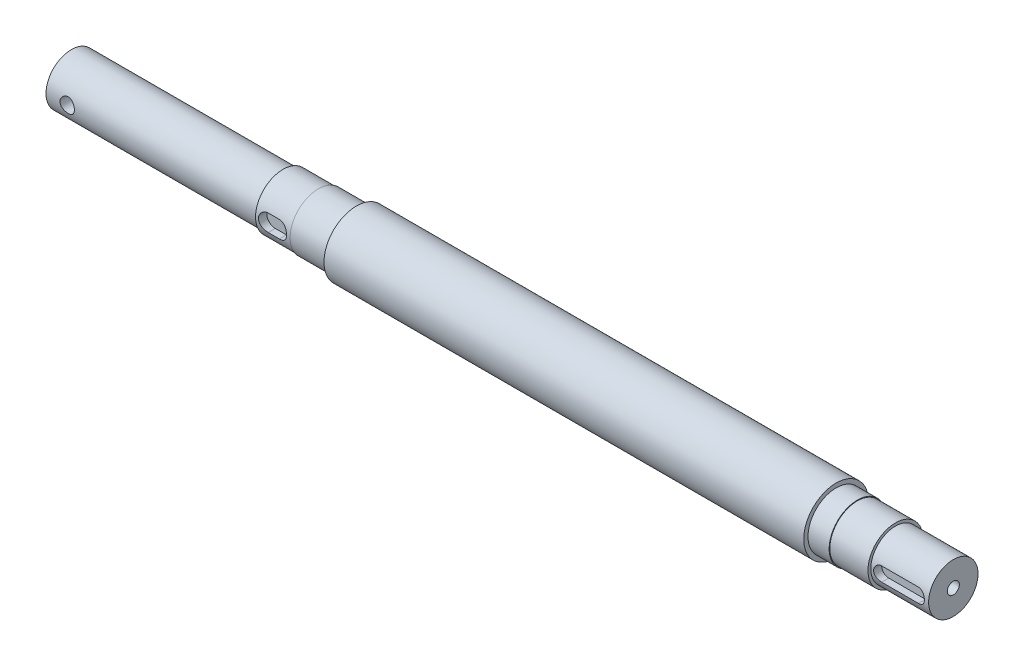
from build123d import *

# Parameters (mm, degrees)
SKETCH_1_R               = 23
EXTRUDE_1_DEPTH          = 340
SKETCH_2_R               = 20
EXTRUDE_2_DEPTH          = 27
SKETCH_3_R               = 19.5
EXTRUDE_3_DEPTH          = 25
EXTRUDE_START            = 15
SKETCH_4_R               = 20
EXTRUDE_4_DEPTH          = 15
EXTRUDE_START_2          = 27
SKETCH_5_R               = 19.5
EXTRUDE_5_DEPTH          = 27
SKETCH_6_R               = 17.5
EXTRUDE_6_DEPTH          = 41
CUT_EXTRUDE_1_DEPTH      = 5.73
SKETCH_8_R               = 18
EXTRUDE_7_DEPTH          = 150
HOLE_WIZARD_M12_2_D      = 10.2
HOLE_WIZARD_M12_2_DEPTH  = 20
HOLE_WIZARD_M12_2_TIP    = 3.064389157
HOLE_WIZARD_M10_1_D      = 8.5
HOLE_WIZARD_M10_1_DEPTH  = 20
HOLE_WIZARD_M10_1_TIP    = 2.553657631
CUT_EXTRUDE_2_DEPTH      = 5
CUT_EXTRUDE_2_DEPTH_BACK = 3.95


with BuildPart() as part:
    # 草图1 → 凸台-拉伸1 (new body)
    with BuildSketch(Plane(origin=(0, 0, 0), x_dir=(0, 0, -1), z_dir=(1, 0, 0))):
        Circle(SKETCH_1_R)
    extrude(amount=EXTRUDE_1_DEPTH)

    # 草图2 → 凸台-拉伸2 (add)
    with BuildSketch(Plane.ZY):
        with Locations(Location((0, 0, 0), (0, 0, 180))):
            Circle(SKETCH_2_R)
    extrude(amount=EXTRUDE_2_DEPTH)

    # 草图3 → 凸台-拉伸3 (add)
    with BuildSketch(Plane.ZY.offset(27)):
        Circle(SKETCH_3_R)
    extrude(amount=EXTRUDE_3_DEPTH)

    # 草图4 → 凸台-拉伸4 (add)
    with BuildSketch(Plane(origin=(340, 0, 0), x_dir=(0, 0, -1), z_dir=(1, 0, 0)).offset(EXTRUDE_START)):
        Circle(SKETCH_4_R)
    extrude(amount=-EXTRUDE_4_DEPTH)

    # 草图5 → 凸台-拉伸5 (add)
    with BuildSketch(Plane(origin=(355, 0, 0), x_dir=(0, 0, -1), z_dir=(1, 0, 0)).offset(EXTRUDE_START_2)):
        with Locations(Location((0, 0, 0), (0, 0, 180))):
            Circle(SKETCH_5_R)
    extrude(amount=-EXTRUDE_5_DEPTH)

    # 草图6 → 凸台-拉伸6 (add)
    with BuildSketch(Plane(origin=(382, 0, 0), x_dir=(0, 0, -1), z_dir=(1, 0, 0))):
        Circle(SKETCH_6_R)
    extrude(amount=EXTRUDE_6_DEPTH)

    # 草图7 → 切除-拉伸1 (cut)
    with BuildSketch(Plane.XY.offset(17.5)):
        with BuildLine():
            Line((389, 5), (415, 5))
            ThreePointArc((415, 5), (420, 0), (415, -5))
            Line((415, -5), (389, -5))
            ThreePointArc((389, -5), (384, 0), (389, 5))
        make_face()
    extrude(amount=-CUT_EXTRUDE_1_DEPTH, mode=Mode.SUBTRACT)

    # 草图8 → 凸台-拉伸7 (add)
    with BuildSketch(Plane.ZY.offset(52)):
        Circle(SKETCH_8_R)
    extrude(amount=EXTRUDE_7_DEPTH)

    # M12 螺纹孔2
    with Locations(Plane.XY.offset(18)):
        with Locations((-187, 0)):
            Hole(HOLE_WIZARD_M12_2_D / 2, depth=HOLE_WIZARD_M12_2_DEPTH)
            with Locations((0, 0, -(HOLE_WIZARD_M12_2_DEPTH + HOLE_WIZARD_M12_2_TIP / 2))):  # 118° drill point
                Cone(0, HOLE_WIZARD_M12_2_D / 2, HOLE_WIZARD_M12_2_TIP, mode=Mode.SUBTRACT)

    # M10 螺纹孔1
    with Locations(Plane(origin=(423, 0, 0), x_dir=(0, 0, -1), z_dir=(1, 0, 0))):
        with Locations((0, 0)):
            Hole(HOLE_WIZARD_M10_1_D / 2, depth=HOLE_WIZARD_M10_1_DEPTH)
            with Locations((0, 0, -(HOLE_WIZARD_M10_1_DEPTH + HOLE_WIZARD_M10_1_TIP / 2))):  # 118° drill point
                Cone(0, HOLE_WIZARD_M10_1_D / 2, HOLE_WIZARD_M10_1_TIP, mode=Mode.SUBTRACT)

    # 草图18 → 切除-拉伸2 (cut, two sides: drawn at the far end of the back side and taken through both)
    with BuildSketch(Plane.XY.offset(17.5).offset(-CUT_EXTRUDE_2_DEPTH_BACK)):
        with BuildLine():
            Line((-36, -6), (-44, -6))
            ThreePointArc((-44, -6), (-50, 0), (-44, 6))
            Line((-44, 6), (-36, 6))
            ThreePointArc((-36, 6), (-30, 0), (-36, -6))
        make_face()
    extrude(amount=CUT_EXTRUDE_2_DEPTH + CUT_EXTRUDE_2_DEPTH_BACK, mode=Mode.SUBTRACT)


solid = part.part
